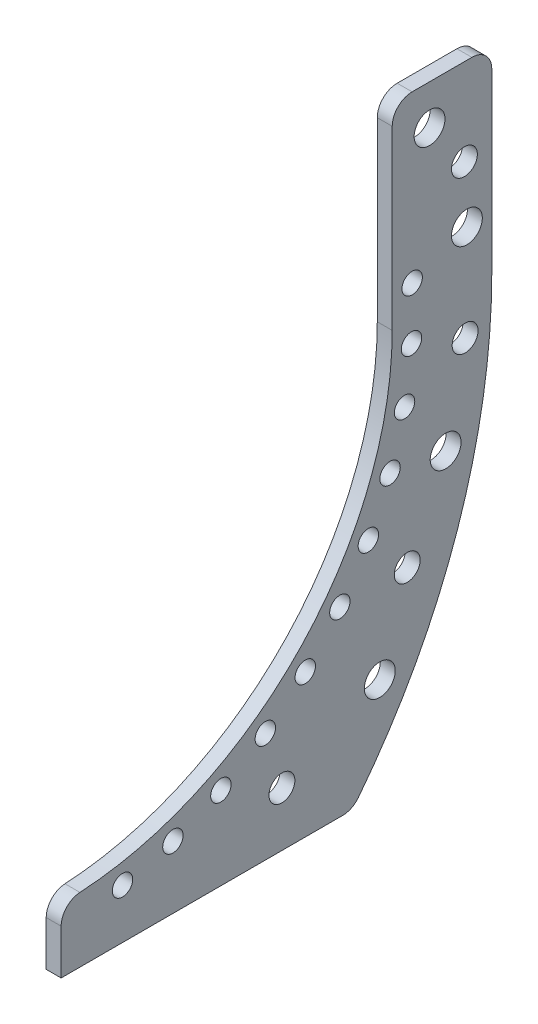
SolidWorks part; units mm, degrees
material "Thornel Mat VMA"
ref_plane "前视基准面" through (0, 0, 0) normal (0, 0, 1) x (1, 0, 0)
ref_plane "上视基准面" through (0, 0, 0) normal (0, 1, 0) x (1, 0, 0)
ref_plane "右视基准面" through (0, 0, 0) normal (1, 0, 0) x (0, 0, -1)
sketch "草图1" plane through (0, 0, 0) normal (1, 0, 0) x (0, 0, -1)
  line L0 (0, 0) -> (0, 48.25) construction
  line L1 (-9.25, 0) -> (-9.25, 19.75)
  line L2 (9.25, 0) -> (9.25, 19.75)
  line L3 (-24, -33.25) -> (-24, -37.75)
  line L4 (9.25, 19.75) -> (19.25, 19.75)
  line L5 (19.25, 19.75) -> (19.25, 0)
  line L6 (-24, -37.75) -> (6.7494, -37.75)
  line L7 (-24, -4.75) -> (-25.4, -4.75)
  line L8 (-25.4, -4.75) -> (-25.4, -14.75)
  line L9 (-25.4, -14.75) -> (-24, -14.75)
  line L10 (-19.25, 0) -> (-19.25, 19.75)
  line L11 (-19.25, 19.75) -> (-9.25, 19.75)
  line L12 (-24, 0) -> (11.1869, -2.1081) construction
  line L13 (-24, 0) -> (10.4888, -7.2859) construction
  line L14 (11.25, 3.1162) -> (11.25, 0) construction
  line L15 (-11.25, 0) -> (-11.25, 3.1162) construction
  line L16 (-24, 0) -> (-11.4381, -2.1822) construction
  line L17 (-24, 0) -> (-13.4117, -7.1029) construction
  line L18 (-24, -33.25) -> (-24, -14.75) construction
  line L19 (14, -37.75) -> (14, -27.25) construction
  line L20 (14, -27.25) -> (19.25, -27.25) construction
  line L21 (-24, 0) -> (-44, 0) construction
  line L22 (11.25, 3.1162) -> (11.1869, -2.1081) construction
  line L23 (10.4888, -7.2859) -> (11.1869, -2.1081) construction
  line L24 (-11.25, 3.1162) -> (-11.4381, -2.1822) construction
  line L25 (-11.4381, -2.1822) -> (-13.4117, -7.1029) construction
  line L26 (-25.4, -9.75) -> (-24, -9.75)
  line L27 (-14.25, 0) -> (-14.25, 19.75)
  line L28 (14.25, 0) -> (14.25, 19.75)
  line L29 (-17.8356, -34.7068) -> (-17.8356, -37.75) construction
  line L30 (-19.25, 19.75) -> (-19.25, 48.25)
  line L31 (-19.25, 48.25) -> (-9.25, 48.25)
  line L32 (19.25, 48.25) -> (19.25, 19.75)
  line L33 (9.25, 19.75) -> (9.25, 48.25)
  line L34 (-9.25, 19.75) -> (-9.25, 48.25)
  line L35 (9.25, 48.25) -> (19.25, 48.25)
  line L36 (-24, 0) -> (-1.8285, -34.25) construction
  line L37 (-24, 0) -> (16.5703, -4.3237) construction
  line L38 (-24, 0) -> (10.7567, -21.3684) construction
  line L39 (16.5703, -4.3237) -> (14.6157, -13.1708) construction
  line L40 (14.6157, -13.1708) -> (10.7567, -21.3684) construction
  line L41 (-14.25, 6.1162) -> (14.25, 6.1162)
  line L42 (5.2389, -39.7) -> (-24, -39.7)
  line L43 (-24, -39.7) -> (-24, -37.75)
  arc A0 (-24, -24) -> (0, 0) centre (-24, 0) ccw construction
  arc A1 (-24, -33.25) -> (9.25, 0) centre (-24, 0) ccw
  arc A2 (-24, -14.75) -> (-9.25, 0) centre (-24, 0) ccw
  arc A3 (5.2389, -39.7) -> (19.25, 0) centre (-44, 0) ccw
  arc A4 (-24, -4.75) -> (-19.25, 0) centre (-24, 0) ccw
  circle A5 centre (11.1869, -2.1081) radius 1.025
  circle A6 centre (10.4888, -7.2859) radius 1.025
  circle A7 centre (9.0331, -12.3036) radius 1.025
  circle A8 centre (6.8516, -17.0511) radius 1.025
  circle A9 centre (3.9925, -21.4239) radius 1.025
  circle A10 centre (0.5183, -25.3262) radius 1.025
  circle A11 centre (-3.4944, -28.672) radius 1.025
  circle A12 centre (-7.9577, -31.388) radius 1.025
  circle A13 centre (11.1869, -2.1081) radius 2.5 construction
  circle A14 centre (10.4888, -7.2859) radius 2.5 construction
  circle A15 centre (11.25, 3.1162) radius 1.025
  circle A16 centre (11.25, 3.1162) radius 2.5 construction
  arc A17 (11.25, 0) -> (-7.9577, -31.388) centre (-24, 0) cw construction
  arc A18 (-11.25, 0) -> (-22.1936, -12.6214) centre (-24, 0) cw construction
  circle A19 centre (-11.4381, -2.1822) radius 1.025
  circle A20 centre (-11.4381, -2.1822) radius 2.5 construction
  circle A21 centre (-13.4117, -7.1029) radius 1.025
  circle A22 centre (-17.2162, -10.7955) radius 1.025
  circle A23 centre (-22.1936, -12.6214) radius 1.025
  circle A25 centre (-11.25, 3.1162) radius 1.025
  circle A26 centre (-11.25, 3.1162) radius 2.5 construction
  circle A27 centre (-13.4117, -7.1029) radius 2.5 construction
  circle A28 centre (8, -29.75) radius 1.55
  circle A29 centre (9.0331, -12.3036) radius 2.5 construction
  circle A30 centre (6.8516, -17.0511) radius 2.5 construction
  circle A31 centre (3.9925, -21.4239) radius 2.5 construction
  circle A32 centre (0.5183, -25.3262) radius 2.5 construction
  circle A33 centre (-3.4944, -28.672) radius 2.5 construction
  circle A34 centre (-7.9577, -31.388) radius 2.5 construction
  circle A35 centre (-17.2162, -10.7955) radius 2.5 construction
  circle A36 centre (-22.1936, -12.6214) radius 2.5 construction
  arc A37 (-24, -9.75) -> (-14.25, 0) centre (-24, 0) ccw
  arc A38 (-24, -38.25) -> (14.25, 0) centre (-24, 0) ccw
  arc A39 (-24, -38.25) -> (14.25, 0) centre (-24, 0) ccw construction
  circle A40 centre (-12.7733, -33.4144) radius 1.025
  circle A41 centre (-17.8356, -34.7068) radius 1.025
  circle A42 centre (-12.7733, -33.4144) radius 2.5 construction
  circle A43 centre (-17.8356, -34.7068) radius 2.5 construction
  circle A44 centre (-21.4, -7.0349) radius 1.3
  circle A45 centre (-16.9174, -2.467) radius 1.55
  arc A48 (-16.9174, -2.467) -> (-21.4, -7.0349) centre (-24, 0) cw construction
  arc A49 (16.5703, -4.3237) -> (-1.8285, -34.25) centre (-24, 0) cw construction
  circle A50 centre (16.5703, -4.3237) radius 1.3
  circle A51 centre (14.6157, -13.1708) radius 1.55
  circle A52 centre (10.7567, -21.3684) radius 1.3
  circle A53 centre (-1.8285, -34.25) radius 1.3
  circle A55 centre (16.75, 5.25) radius 1.55
  circle A56 centre (-16.75, 5.25) radius 1.55
  circle A57 centre (-13, 15.75) radius 1.55
  circle A58 centre (-16.5, 11.05) radius 1.3
  circle A59 centre (13, 15.75) radius 1.55
  circle A60 centre (16.5, 11.05) radius 1.3
  dimension "D1" = 24
  dimension "D2" = 18.5
  dimension "D4" = 10
  dimension "D5" = 1.4
  dimension "D6" = 10
  dimension "D8" = 2.05
  dimension "D10" = 5
  dimension "D11" = 4
  dimension "D13" = 12.75
  dimension "D15" = 3.5
  dimension "D16" = 3.1
  dimension "D18" = 6
  dimension "D23" = 53
  dimension "D24" = 2.6
  dimension "D25" = 3.1
  dimension "D26" = 7.5
  dimension "D33" = 40.8
  dimension "D28" = 6.4
  dimension "D34" = 26
  dimension "D3" = 4.5
  dimension "D7" = 8.5
  dimension "D9" = 35.25
  dimension "D12" = 24
  dimension "D14" = 24.5
  dimension "D17" = 8
  dimension "D19" = 2.5
  dimension "D20" = 20
  dimension "D21" = 5
  dimension "D27" = 4
  dimension "D29" = 2.5
  dimension "D30" = 14.5
  dimension "D31" = 32
  dimension "D32" = 1.95
  dimension "D35" = 51
  dimension "D36" = 3
  dimension "D37" = 33
  dimension "D38" = 5.8
  dimension "D39" = 4
  dimension "D22" = 5
extrude "凸台-拉伸1" add sketch "草图1" along normal blind 1.5 contours A38 L6 A3 L5 L4 L28 A55 A53 A52 A51 A50 A28 | L2 L41 L28 L4 | L42 A3 L6 L43 | L6 A38 L28 L41 L2 A1 L3 A41 A40 A5 A6 A7 A8 A9 A10 A11 A12 A15 | L43 A38 L6
fillet "R2 圆角1" radius 2 4 edges at (0.75, 19.75, -19.25) (0.75, 19.75, -9.25) (0.75, -33.25, 24) (0.75, -39.7, -5.2389)
